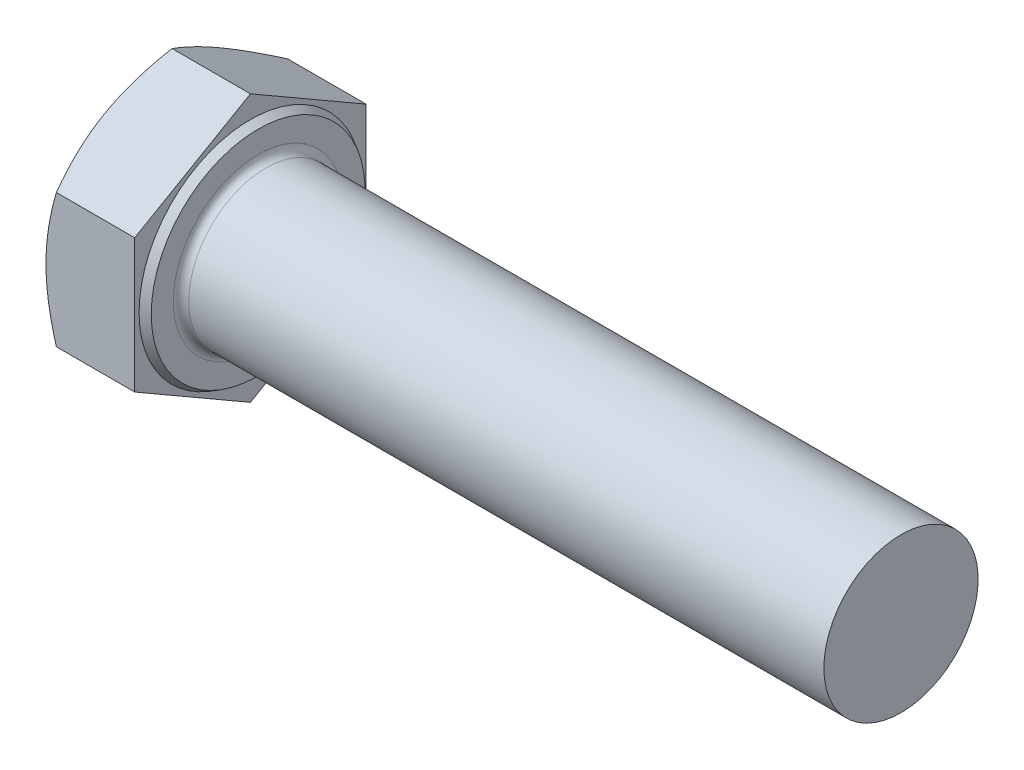
from build123d import *

# Parameters (mm, degrees)
EXTRUDE_387_DEPTH = 7.5
FILLET_1280_R     = 0.6


with BuildPart() as part:
    # 草图1 → Extrude 387 (new body)
    with BuildSketch(Plane(origin=(0, 0, 0), x_dir=(0, 0, -1), z_dir=(1, 0, 0))):
        Polygon((9, 5.196152423), (9, -5.196152423), (0, -10.392304845), (-9, -5.196152423), (-9, 5.196152423), (0, 10.392304845), align=None)
    extrude(amount=EXTRUDE_387_DEPTH)

    # 草图2 → 凸台-旋转1 (revolve)
    with BuildSketch(Plane.XY, mode=Mode.PRIVATE) as revolve_1_sk:
        Polygon((0, 0), (57.5, 0), (57.5, 4.4845), (57.5, 6), (27.5, 6), (0, 6), align=None)
    revolve(revolve_1_sk.sketch.rotate(Axis((0, 0, 0), (1, 0, 0)), 90), axis=Axis((0, 0, 0), (1, 0, 0)))

    # 草图3 → 切除-旋转1 (revolve, cut)
    with BuildSketch(Plane.XY):
        Polygon((0, 9), (3.690598923, 15.392304845), (3.690598923, 20.392304845), (-10, 20.392304845), (-10, 9), align=None)
    revolve(axis=Axis((0, 0, 0), (1, 0, 0)), mode=Mode.SUBTRACT)

    # 草图4 → 切除-旋转3 (revolve, cut)
    with BuildSketch(Plane.XY, mode=Mode.PRIVATE) as cut_revolve_3_sk:
        Polygon((7.5, 8.315), (6.9, 8.661410162), (6.9, 10.392304845), (7.5, 10.392304845), align=None)
    revolve(cut_revolve_3_sk.sketch.rotate(Axis((0, 0, 0), (1, 0, 0)), 90), axis=Axis((0, 0, 0), (1, 0, 0)), mode=Mode.SUBTRACT)

    # Fillet 1280
    fillet_1280_edges = [part.edges().sort_by_distance(p)[0] for p in [
        (7.5, 0, -6),
    ]]
    fillet(fillet_1280_edges, radius=FILLET_1280_R)


solid = part.part
